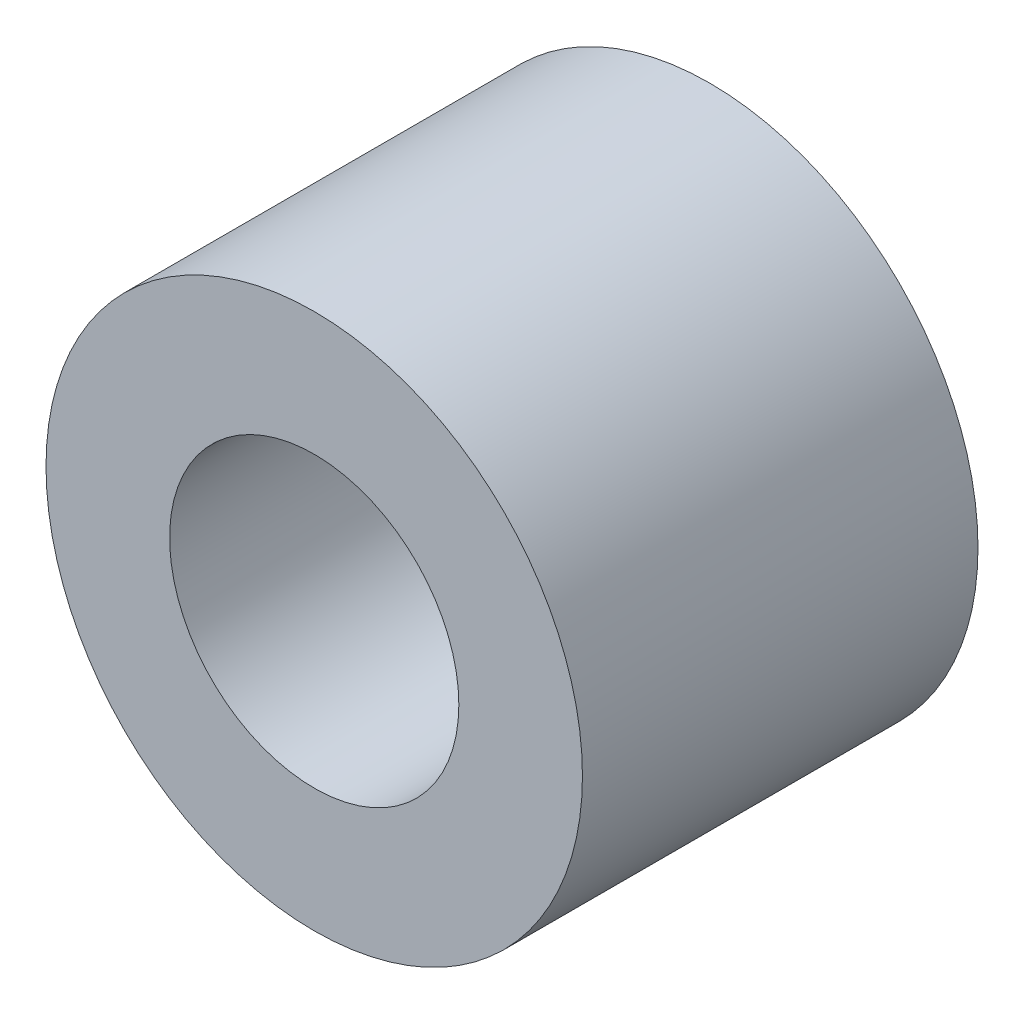
SolidWorks part; units mm, degrees
ref_plane "Front Plane" through (0, 0, 0) normal (0, 0, 1) x (1, 0, 0)
ref_plane "Top Plane" through (0, 0, 0) normal (0, 1, 0) x (1, 0, 0)
ref_plane "Right Plane" through (0, 0, 0) normal (1, 0, 0) x (0, 0, -1)
sketch "Sketch1" plane through (0, 0, 0) normal (0, 0, 1) x (1, 0, 0)
  circle A0 centre (0, 0) radius 10.85
  circle A1 centre (0, 0) radius 5.85
extrude "Boss-Extrude1" add sketch "Sketch1" along normal blind 16
